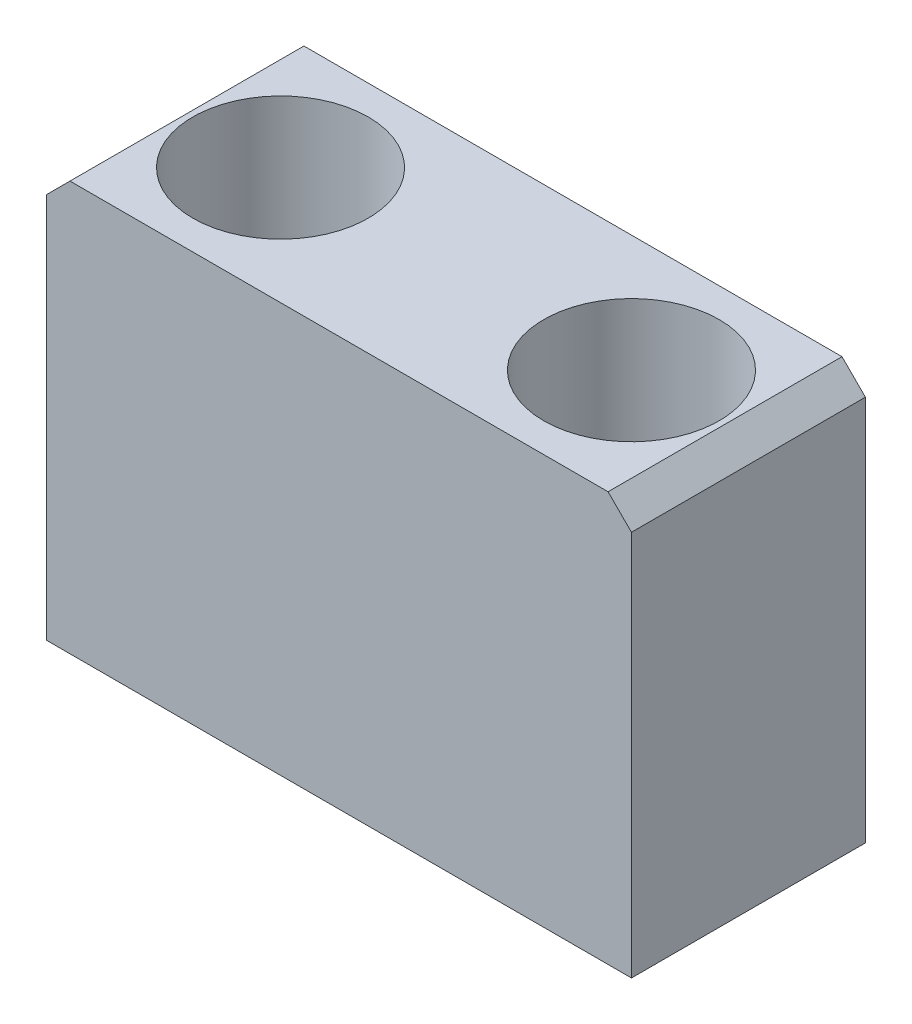
from build123d import *

# Parameters (mm, degrees)
SKETCH_2_W                   = 50
SKETCH_2_H                   = 35
EXTRUDE_1_DEPTH              = 10
HOLE_WIZARD_M8_1_D           = 9
HOLE_WIZARD_M8_1_CBORE_D     = 15
HOLE_WIZARD_M8_1_CBORE_DEPTH = 15
CHAMFER_1_SIZE               = 2


with BuildPart() as part:
    # 草图2 → 凸台-拉伸1 (new, symmetric)
    with BuildSketch(Plane.XY):
        Rectangle(SKETCH_2_W, SKETCH_2_H)
    extrude(amount=EXTRUDE_1_DEPTH, both=True)

    # M8 六角凹头螺钉的柱形沉头孔1 (through all)
    with Locations(Plane(origin=(0, 17.5, 0), x_dir=(1, 0, 0), z_dir=(0, 1, 0))):
        with Locations((15, 0), (-15, 0)):
            CounterBoreHole(HOLE_WIZARD_M8_1_D / 2, HOLE_WIZARD_M8_1_CBORE_D / 2, HOLE_WIZARD_M8_1_CBORE_DEPTH)

    # 倒角1
    chamfer_1_edges = [part.edges().sort_by_distance(p)[0] for p in [
        (-25, 17.5, 0),
        (25, 17.5, 0),
    ]]
    chamfer(chamfer_1_edges, length=CHAMFER_1_SIZE)


solid = part.part
